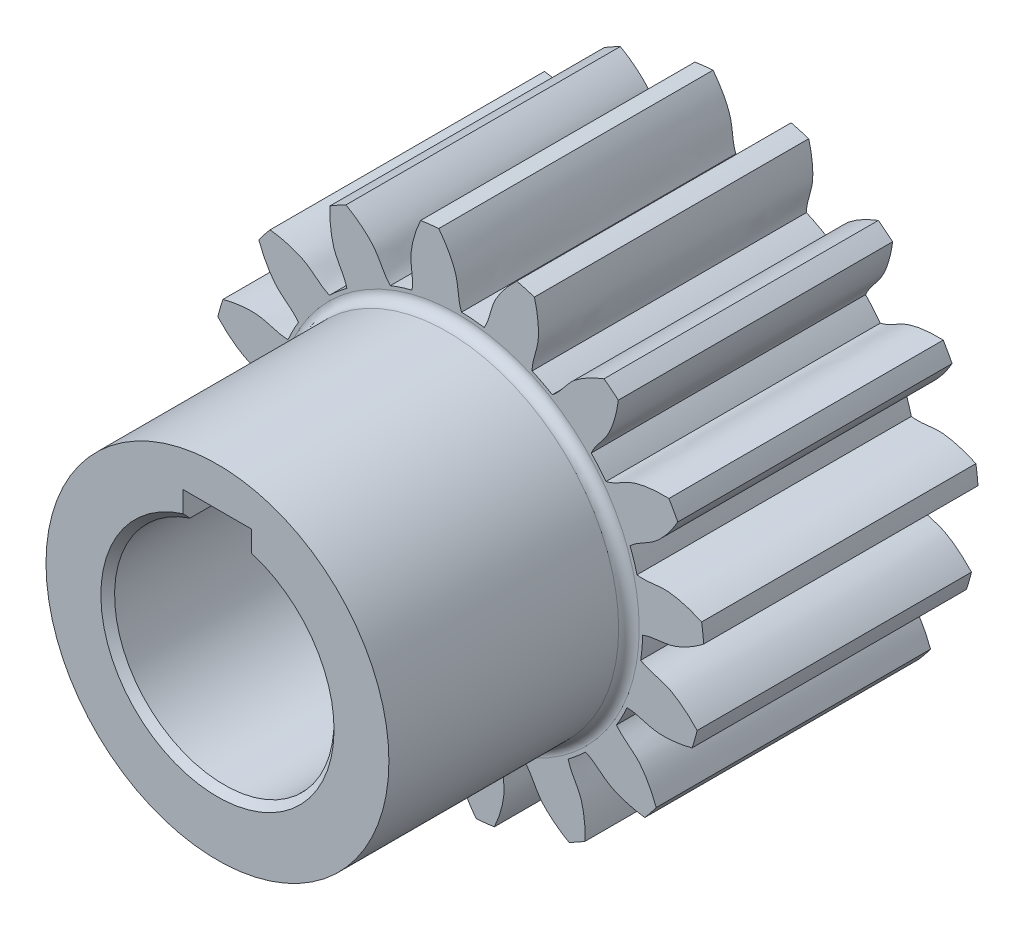
SolidWorks part; units mm, degrees
material "Q235B"
ref_plane "Front Plane" through (0, 0, 0) normal (0, 0, 1) x (1, 0, 0)
ref_plane "Top Plane" through (0, 0, 0) normal (0, 1, 0) x (1, 0, 0)
ref_plane "Right Plane" through (0, 0, 0) normal (1, 0, 0) x (0, 0, -1)
sketch "Sketch1" plane through (0, 0, 0) normal (0, 0, 1) x (1, 0, 0)
  circle A0 centre (0, 0) radius 27
  circle A1 centre (0, 0) radius 16
extrude "Boss-Extrude1" add sketch "Sketch1" along normal blind 40
sketch "Sketch2" plane through (0, 0, 0) normal (0, 0, 1) x (1, 0, 0)
  arc A0 (35.5954, 5.382) -> (35.8958, 2.7368) centre (0, 0) cw
  arc A1 (26.1742, 6.6267) -> (26.9936, -0.5888) centre (0, 0) cw
  spline S0 degree 3 poles (35.8958, 2.7368) (35.1715, 2.179) (34.0472, 1.4205) (32.4583, 0.6444) (30.3015, -0.1856) (28.3432, -0.038) (26.9936, -0.5888) knots 0 0 0 0 0.284727 0.4198 0.549994 1 1 1 1
  spline S1 degree 3 poles (35.5954, 5.382) (34.7645, 5.7632) (33.4987, 6.2503) (31.7762, 6.6503) (29.4882, 6.9756) (27.613, 6.3926) (26.1742, 6.6267) knots 0 0 0 0 0.284727 0.4198 0.549994 1 1 1 1
extrude "Boss-Extrude2" add sketch "Sketch2" along normal blind 40
pattern_circular "CirPattern1" count 16 over 360 about axis through (0, 0, 40) along (0, 0, -1) of "Boss-Extrude2"
sketch "Sketch3" plane through (0, 0, 40) normal (0, 0, 1) x (1, 0, 0)
  circle A0 centre (0, 0) radius 25
  circle A1 centre (0, 0) radius 16 construction
  circle A2 centre (0, 0) radius 16
  dimension "D1" = 50
extrude "Boss-Extrude3" add sketch "Sketch3" along normal blind 35
fillet "Fillet1" radius 1.5 1 edges at (25, 0, 40)
sketch "Sketch4" plane through (0, 0, 0) normal (0, 0, -1) x (-1, 0, 0)
  circle A0 centre (0, 0) radius 21
  dimension "D1" = 42
extrude "Cut-Extrude1" cut sketch "Sketch4" against normal blind 8
chamfer "Chamfer1" distance 1 angle 45 3 edges at (-16, 0, 8) (16, 0, 75) (-21, 0, 0)
sketch "Sketch5" plane through (0, 0, 75) normal (0, 0, 1) x (1, 0, 0)
  line L1 (5, 12.7) -> (-5, 12.7)
  line L2 (5, 12.7) -> (5, 19.3)
  line L3 (5, 19.3) -> (-5, 19.3)
  line L4 (-5, 12.7) -> (-5, 19.3)
  line L5 (5, 12.7) -> (-5, 19.3) construction
  line L6 (5, 19.3) -> (-5, 12.7) construction
  circle A0 centre (0, 0) radius 16 construction
  point P0 (0, 16)
  dimension "D1" = 10
  dimension "D2" = 19.3
extrude "Cut-Extrude2" cut sketch "Sketch5" against normal up to next
